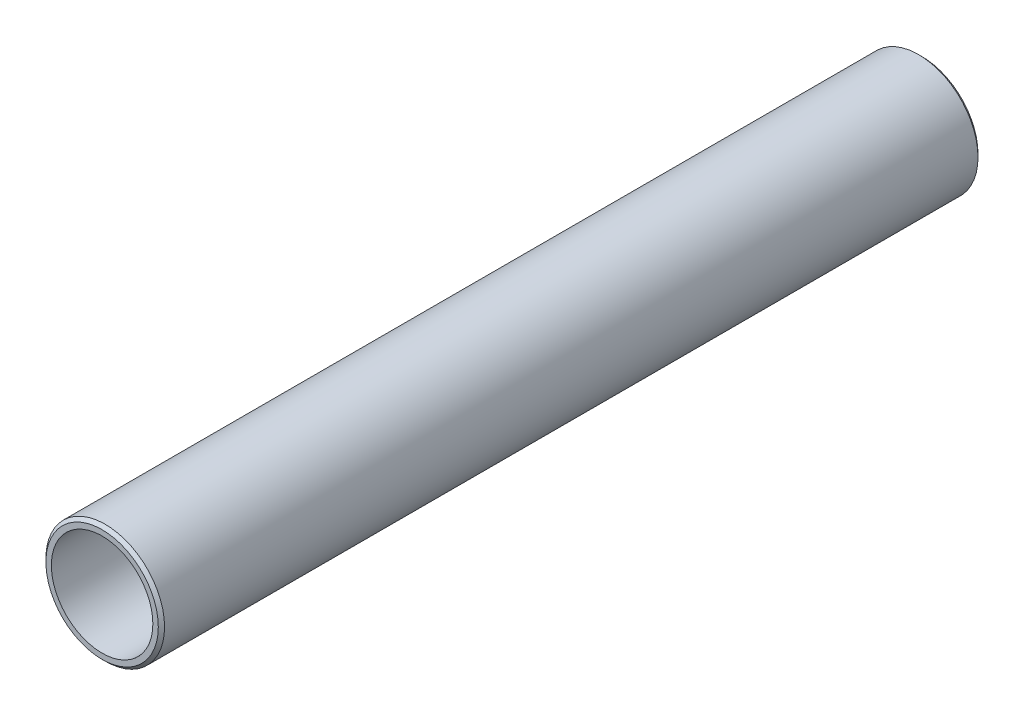
SolidWorks part; units mm, degrees
material "普通碳钢"
ref_plane "前视基准面" through (0, 0, 0) normal (0, 0, 1) x (1, 0, 0)
ref_plane "上视基准面" through (0, 0, 0) normal (0, 1, 0) x (1, 0, 0)
ref_plane "右视基准面" through (0, 0, 0) normal (1, 0, 0) x (0, 0, -1)
sketch "草图1" plane through (0, 0, 0) normal (0, 0, 1) x (1, 0, 0)
  circle A0 centre (0, 0) radius 38
  circle A1 centre (0, 0) radius 32.5
  dimension "D1" = 76
  dimension "D2" = 65
extrude "凸台-拉伸1" add sketch "草图1" along normal blind 525
chamfer "倒角1" distance 2 angle 45 2 edges at (38, 0, 525) (38, 0, 0)
